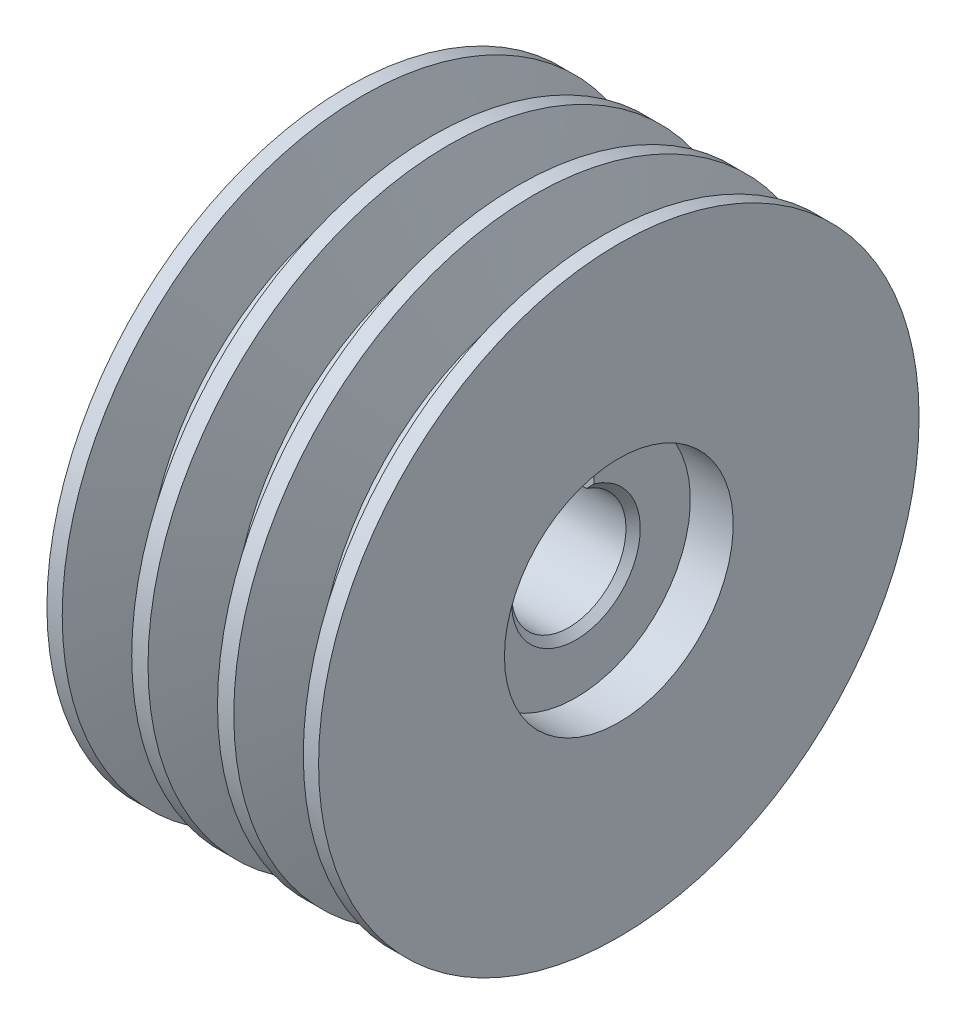
SolidWorks part; units mm, degrees
ref_plane "前视基准面" through (0, 0, 0) normal (0, 0, 1) x (1, 0, 0)
ref_plane "上视基准面" through (0, 0, 0) normal (0, 1, 0) x (1, 0, 0)
ref_plane "右视基准面" through (0, 0, 0) normal (1, 0, 0) x (0, 0, -1)
sketch "草图1" plane through (0, 0, 0) normal (0, 0, 1) x (1, 0, 0)
  line L0 (0, 0) -> (64.8368, 0) construction
  line L1 (0, 8) -> (0, 42)
  line L2 (0, 42) -> (38, 42)
  line L3 (38, 42) -> (38, 16)
  line L4 (38, 16) -> (32, 16)
  line L5 (32, 16) -> (32, 8)
  line L6 (32, 8) -> (0, 8)
  line L7 (2.1385, 42) -> (4.8901, 33) construction
  line L8 (4.8901, 33) -> (9.1099, 33) construction
  line L9 (9.1099, 33) -> (11.8615, 42) construction
  line L10 (0, 40) -> (38, 40) construction
  line L11 (7, 33) -> (7, 8) construction
  point P17 (2.75, 40)
  point P18 (11.25, 40)
  dimension "d2" = 84
  dimension "L" = 32
  dimension "B" = 38
  dimension "d" = 16
  dimension "d1" = 32
  dimension "dd" = 80
  dimension "f" = 7
  dimension "槽轮角" = 34
  dimension "bd" = 8.5
  dimension "hf" = 7
  dimension "ha" = 2
revolve "旋转1" add sketch "草图1" angle 360 about L0
sketch "草图2" plane through (0, 0, 0) normal (0, 0, 1) x (1, 0, 0)
  line L0 (9.1099, 33) -> (11.8615, 42) construction
  line L1 (4.8901, 33) -> (9.1099, 33) construction
  line L2 (2.1385, 42) -> (4.8901, 33) construction
  line L3 (9.1099, 33) -> (11.8615, 42)
  line L4 (4.8901, 33) -> (9.1099, 33)
  line L5 (2.1385, 42) -> (4.8901, 33)
  line L6 (2.1385, 42) -> (11.8615, 42)
  line L7 (0, 0) -> (38, 0) construction
  line L8 (38, -16) -> (38, 16) construction
revolve "切除-旋转1" cut sketch "草图2" angle 360 about L7
pattern_linear "阵列(线性)1" count 3 spacing 12 along (1, 0, 0) of "切除-旋转1"
chamfer "倒角1" distance 1 2 edges at (32, 0, 8) (0, 0, 8)
sketch "草图4" plane through (0, 0, 0) normal (-1, 0, 0) x (0, 0, 1)
  line L1 (-2.5, 7.5993) -> (2.5, 7.5993)
  line L2 (-2.5, 7.5993) -> (-2.5, 10.3)
  line L3 (-2.5, 10.3) -> (2.5, 10.3)
  line L4 (2.5, 7.5993) -> (2.5, 10.3)
  circle A0 centre (0, 0) radius 8 construction
  point P6 (0.2, 10.3)
  dimension "键槽高度" = 10.3
  dimension "键槽宽度" = 5
  dimension "t1" = 2.3
extrude "切除-拉伸1" cut sketch "草图4" against normal through all
